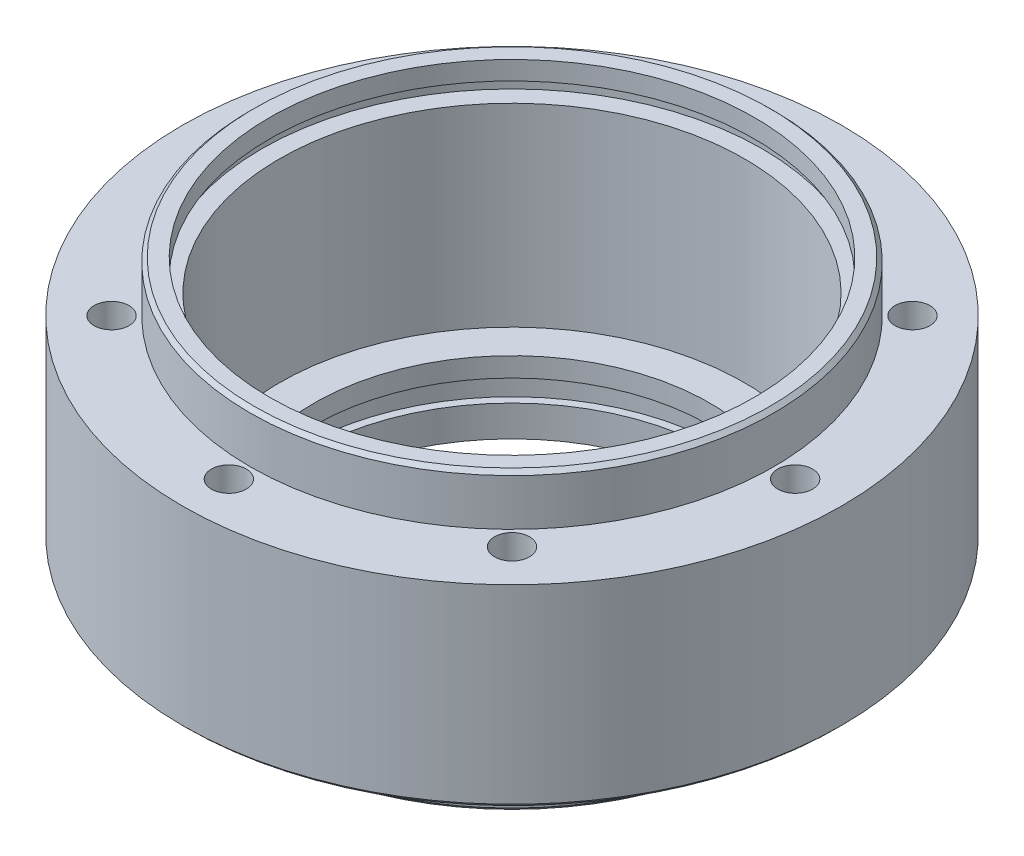
from build123d import *

# Parameters (mm, degrees)
SKETCH1_R                                          = 85
BOSS_EXTRUDE1_DEPTH                                = 50
SKETCH2_R                                          = 67.5
BOSS_EXTRUDE2_DEPTH                                = 13
SKETCH3_R                                          = 65
BOSS_EXTRUDE3_DEPTH                                = 15
CHAMFER1_SIZE                                      = 1
SKETCH4_R                                          = 52.5
CUT_EXTRUDE1_DEPTH                                 = 55
SKETCH5_R                                          = 51
CUT_EXTRUDE2_DEPTH                                 = 133.193040664
CUT_EXTRUDE3_START                                 = -8
SKETCH6_R                                          = 55
CUT_EXTRUDE3_DEPTH                                 = 8.5
HOLE_SIZE_BASED_ON_SOCKET_HEAD_CAP_SCR_D           = 9
HOLE_SIZE_BASED_ON_SOCKET_HEAD_CAP_SCR_CBORE_D     = 15
HOLE_SIZE_BASED_ON_SOCKET_HEAD_CAP_SCR_CBORE_DEPTH = 30
CIRPATTERN1_COUNT                                  = 8
CHAMFER2_SIZE                                      = 1
SKETCH15_R                                         = 55
SKETCH15_R_2                                       = 51
BOSS_EXTRUDE4_DEPTH                                = 1.5
CIRPATTERN3_COUNT                                  = 8
SKETCH20_R                                         = 53
CUT_EXTRUDE8_DEPTH                                 = 8
SKETCH22_R                                         = 60
CUT_EXTRUDE11_DEPTH                                = 58
CUT_EXTRUDE12_START                                = -8
SKETCH23_R                                         = 64.5
CUT_EXTRUDE12_DEPTH                                = 3.2
SKETCH25_R                                         = 62.5
CUT_EXTRUDE13_DEPTH                                = 8


with BuildPart() as part:
    # Sketch1 → Boss-Extrude1 (new body)
    with BuildSketch(Plane(origin=(0, 0, 0), x_dir=(1, 0, 0), z_dir=(0, 1, 0))):
        with Locations(Location((0, 0, 0), (0, 0, 270))):
            Circle(SKETCH1_R)
    extrude(amount=BOSS_EXTRUDE1_DEPTH)

    # Sketch2 → Boss-Extrude2 (add)
    with BuildSketch(Plane(origin=(0, 50, 0), x_dir=(1, 0, 0), z_dir=(0, 1, 0))):
        with Locations(Location((0, 0, 0), (0, 0, 270))):
            Circle(SKETCH2_R)
    extrude(amount=BOSS_EXTRUDE2_DEPTH)

    # Sketch3 → Boss-Extrude3 (add)
    with BuildSketch(Plane.XZ):
        with Locations(Location((0, 0, 0), (0, 0, 90))):
            Circle(SKETCH3_R)
    extrude(amount=BOSS_EXTRUDE3_DEPTH)

    # Chamfer1
    chamfer1_edges = [part.edges().sort_by_distance(p)[0] for p in [
        (0, -15, -65),
        (0, 63, -67.5),
    ]]
    chamfer(chamfer1_edges, length=CHAMFER1_SIZE)

    # Sketch4 → Cut-Extrude1 (cut)
    with BuildSketch(Plane(origin=(0, 63, 0), x_dir=(1, 0, 0), z_dir=(0, 1, 0))):
        with Locations(Location((0, 0, 0), (0, 0, 270))):
            Circle(SKETCH4_R)
    extrude(amount=-CUT_EXTRUDE1_DEPTH, mode=Mode.SUBTRACT)

    # Sketch5 → Cut-Extrude2 (cut, through all)
    with BuildSketch(Plane(origin=(0, 8, 0), x_dir=(1, 0, 0), z_dir=(0, 1, 0))):
        with Locations(Location((0, 0, 0), (0, 0, 270))):
            Circle(SKETCH5_R)
    extrude(amount=-CUT_EXTRUDE2_DEPTH, mode=Mode.SUBTRACT)

    # Sketch6 → Cut-Extrude3 (cut)
    with BuildSketch(Plane.XZ.offset(15).offset(CUT_EXTRUDE3_START)):
        with Locations(Location((0, 0, 0), (0, 0, 270))):
            Circle(SKETCH6_R)
    extrude(amount=-CUT_EXTRUDE3_DEPTH, mode=Mode.SUBTRACT)

    # Hole size (% based on socket head cap screw type)1 (through all)
    with Locations(Plane(origin=(0, 0, 0), x_dir=(-1, 0, 0), z_dir=(0, -1, 0))):
        with Locations((0, 73)):
            hole_size_based_on_socket_head_cap_scr = CounterBoreHole(HOLE_SIZE_BASED_ON_SOCKET_HEAD_CAP_SCR_D / 2, HOLE_SIZE_BASED_ON_SOCKET_HEAD_CAP_SCR_CBORE_D / 2, HOLE_SIZE_BASED_ON_SOCKET_HEAD_CAP_SCR_CBORE_DEPTH)

    # CirPattern1: Hole size (% based on socket head cap screw type)1 ×8 about axis
    cirpattern1_axis = Axis((0, 0, 0), (0, 1, 0))
    for i in range(1, CIRPATTERN1_COUNT):
        add(hole_size_based_on_socket_head_cap_scr.rotate(cirpattern1_axis, i * 360 / CIRPATTERN1_COUNT), mode=Mode.SUBTRACT)

    # Chamfer2
    chamfer2_edges = [part.edges().sort_by_distance(p)[0] for p in [
        (0, 0, -85),
    ]]
    chamfer(chamfer2_edges, length=CHAMFER2_SIZE)

    # Sketch15 → Boss-Extrude4 (add)
    with BuildSketch(Plane.XZ.offset(-1.5)):
        with Locations(Location((0, 0, 0), (0, 0, 270))):
            Circle(SKETCH15_R)
        with Locations(Location((0, 0, 0), (0, 0, 90))):
            Circle(SKETCH15_R_2, mode=Mode.SUBTRACT)
    extrude(amount=BOSS_EXTRUDE4_DEPTH)

    # Sketch19 → M8 Tapped Hole1 (revolve, cut)
    with BuildSketch(Plane(origin=(-27.935890563, 0, 67.443205873), x_dir=(0, 0, -1), z_dir=(1, 0, 0))):
        Polygon((0, 0), (0, 25.792926105), (3.4, 23.75), (3.4, 0), align=None)
    m8_tapped_hole1 = revolve(axis=Axis((-27.935890563, -6.35, 67.443205873), (0, 1, 0)), mode=Mode.SUBTRACT)

    # CirPattern3: M8 Tapped Hole1 ×8 about axis
    cirpattern3_axis = Axis((0, 0, 0), (0, 1, 0))
    for i in range(1, CIRPATTERN3_COUNT):
        add(m8_tapped_hole1.rotate(cirpattern3_axis, i * 360 / CIRPATTERN3_COUNT), mode=Mode.SUBTRACT)

    # Sketch20 → Cut-Extrude8 (cut)
    with BuildSketch(Plane.XZ.offset(15)):
        with Locations(Location((0, 0, 0), (0, 0, 270))):
            Circle(SKETCH20_R)
    extrude(amount=-CUT_EXTRUDE8_DEPTH, mode=Mode.SUBTRACT)

    # Sketch22 → Cut-Extrude11 (cut)
    with BuildSketch(Plane(origin=(0, 63, 0), x_dir=(1, 0, 0), z_dir=(0, 1, 0))):
        with Locations(Location((0, 0, 0), (0, 0, 270))):
            Circle(SKETCH22_R)
    extrude(amount=-CUT_EXTRUDE11_DEPTH, mode=Mode.SUBTRACT)

    # Sketch23 → Cut-Extrude12 (cut)
    with BuildSketch(Plane(origin=(0, 63, 0), x_dir=(1, 0, 0), z_dir=(0, 1, 0)).offset(CUT_EXTRUDE12_START)):
        with Locations(Location((0, 0, 0), (0, 0, 270))):
            Circle(SKETCH23_R)
    extrude(amount=CUT_EXTRUDE12_DEPTH, mode=Mode.SUBTRACT)

    # Sketch25 → Cut-Extrude13 (cut)
    with BuildSketch(Plane(origin=(0, 63, 0), x_dir=(1, 0, 0), z_dir=(0, 1, 0))):
        with Locations(Location((0, 0, 0), (0, 0, 270))):
            Circle(SKETCH25_R)
    extrude(amount=-CUT_EXTRUDE13_DEPTH, mode=Mode.SUBTRACT)


solid = part.part
